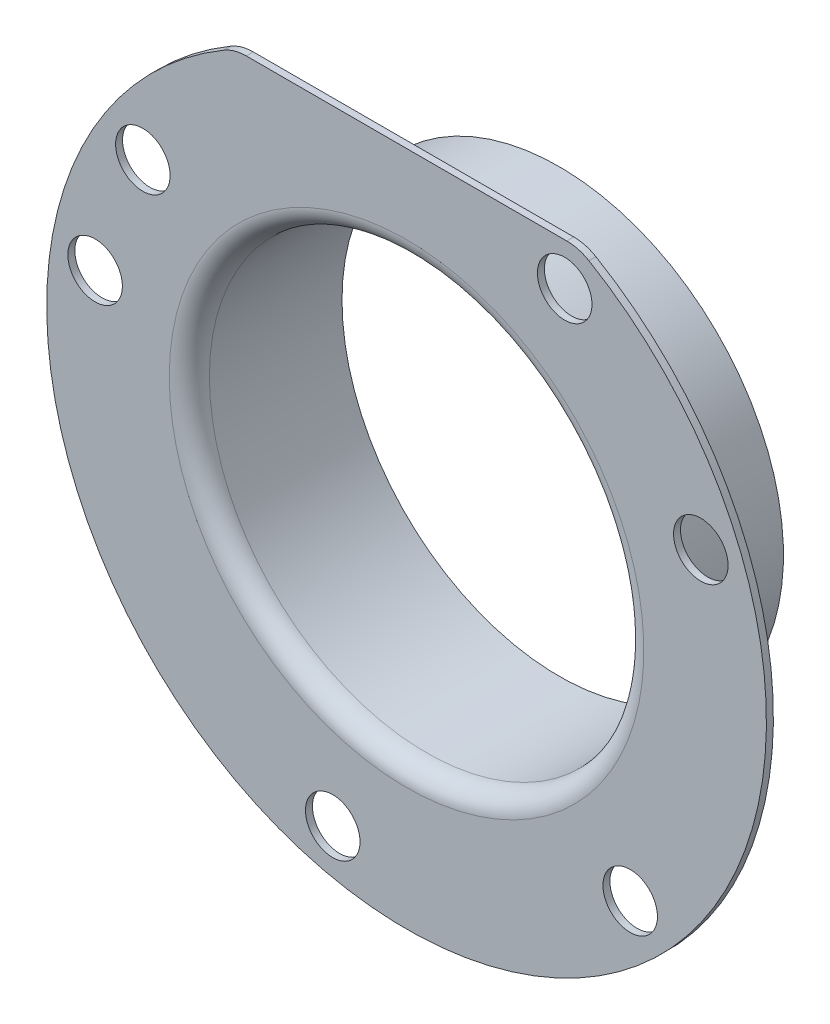
SolidWorks part; units mm, degrees
material "SPHC"
ref_plane "Front Plane" through (0, 0, 0) normal (0, 0, 1) x (1, 0, 0)
ref_plane "Top Plane" through (0, 0, 0) normal (0, 1, 0) x (1, 0, 0)
ref_plane "Right Plane" through (0, 0, 0) normal (1, 0, 0) x (0, 0, -1)
sketch "Sketch1" plane through (0, 0, 0) normal (1, 0, 0) x (0, 0, -1)
  line L0 (0, 0) -> (-35, 0) construction
  line L1 (0, 49.8) -> (-30.4, 49.8)
  line L2 (-35, 54.4) -> (-35, 82.5)
  arc A0 (-30.4, 49.8) -> (-35, 54.4) centre (-30.4, 54.4) cw
  point P9 (-35, 49.8)
  dimension "D4" = 4.6
  dimension "D1" = 35
  dimension "D2" = 99.6
  dimension "D3" = 165
revolve "Revolve-Thin2" add sketch "Sketch1" angle 360 about L0
sketch "Sketch2" plane through (0, 0, 35) normal (0, 0, 1) x (1, 0, 0)
  line L0 (0, 0) -> (-60.4567, 40.0154) construction
  line L1 (0, 0) -> (72.5, 0) construction
  line L2 (0, 0) -> (36.25, 62.7868) construction
  line L3 (0, 0) -> (67.4553, 26.5713) construction
  line L4 (0, 0) -> (51.2652, -51.2652) construction
  line L5 (0, 0) -> (-16.9248, -70.4968) construction
  line L6 (0, 0) -> (-71.3986, 12.5895) construction
  line L7 (-45, 72.5) -> (45, 72.5)
  line L8 (45, 72.5) -> (45, 84.5)
  line L9 (45, 84.5) -> (-45, 84.5)
  line L10 (-45, 84.5) -> (-45, 72.5)
  circle A0 centre (0, 0) radius 72.5 construction
  circle A1 centre (-60.4567, 40.0154) radius 6.25
  circle A2 centre (36.25, 62.7868) radius 6.25
  circle A3 centre (67.4553, 26.5713) radius 6.25
  circle A4 centre (51.2652, -51.2652) radius 6.25
  circle A5 centre (-16.9248, -70.4968) radius 6.25
  circle A6 centre (-71.3986, 12.5895) radius 6.25
  dimension "D1" = 145
  dimension "D2" = 12.5
  dimension "D3" = 21.5
  dimension "D4" = 45
  dimension "D5" = 125
  dimension "D6" = 145
  dimension "D7" = 110
  dimension "D8" = 110
  dimension "D9" = 125
  dimension "D10" = 72.5
  dimension "D11" = 12
  dimension "D12" = 90
  dimension "D13" = 45
extrude "Cut-Extrude1" cut sketch "Sketch2" against normal up to next
fillet "Fillet1" radius 10 2 edges at (-39.37, 72.5, 34.2) (39.37, 72.5, 34.2)
ref_plane "Plane1" through (0, 0, 0) normal (-0.7071, 0.7071, 0) x (0.7071, 0.7071, 0)
sketch "Sketch3" plane through (0, 0, 0) normal (-0.7071, 0.7071, 0) x (0.7071, 0.7071, 0)
  circle A0 centre (0, -10) radius 2.75
  dimension "D1" = 5.5
  dimension "D2" = 10
extrude "Cut-Extrude2" [suppressed] cut sketch "Sketch3" against normal through all
pattern_circular "CirPattern1" [suppressed] count 3 over 360
